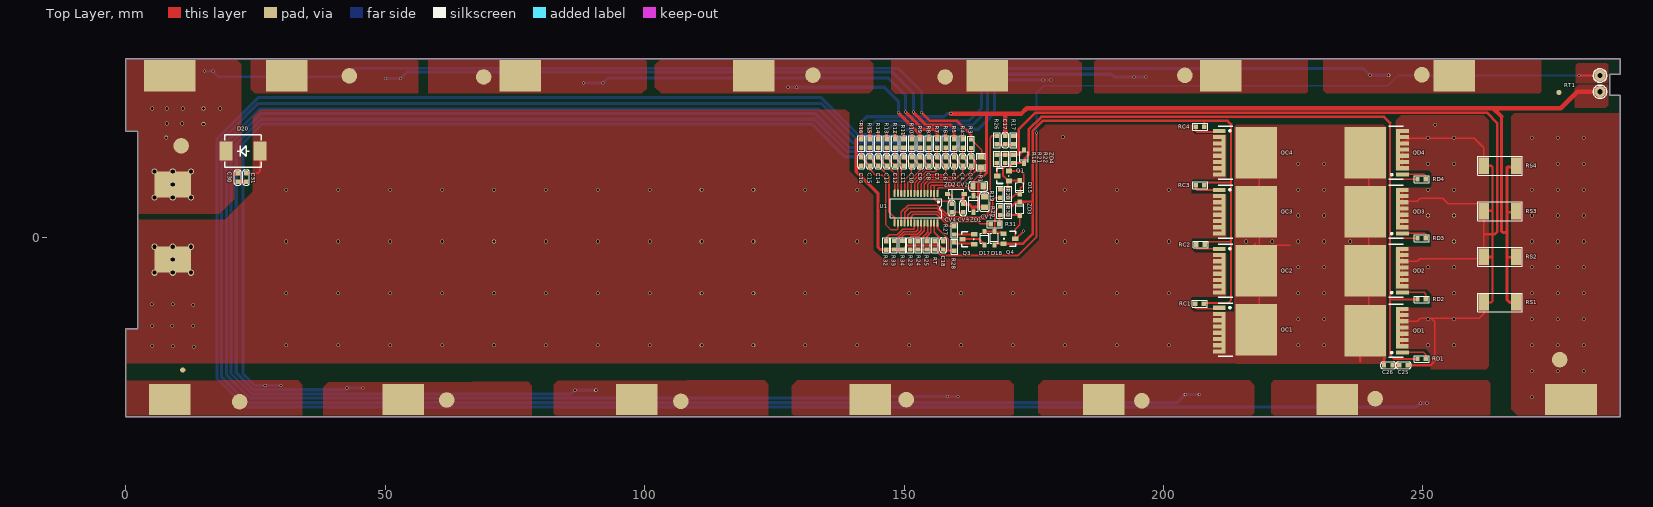
[diagram p0: Top Layer view]
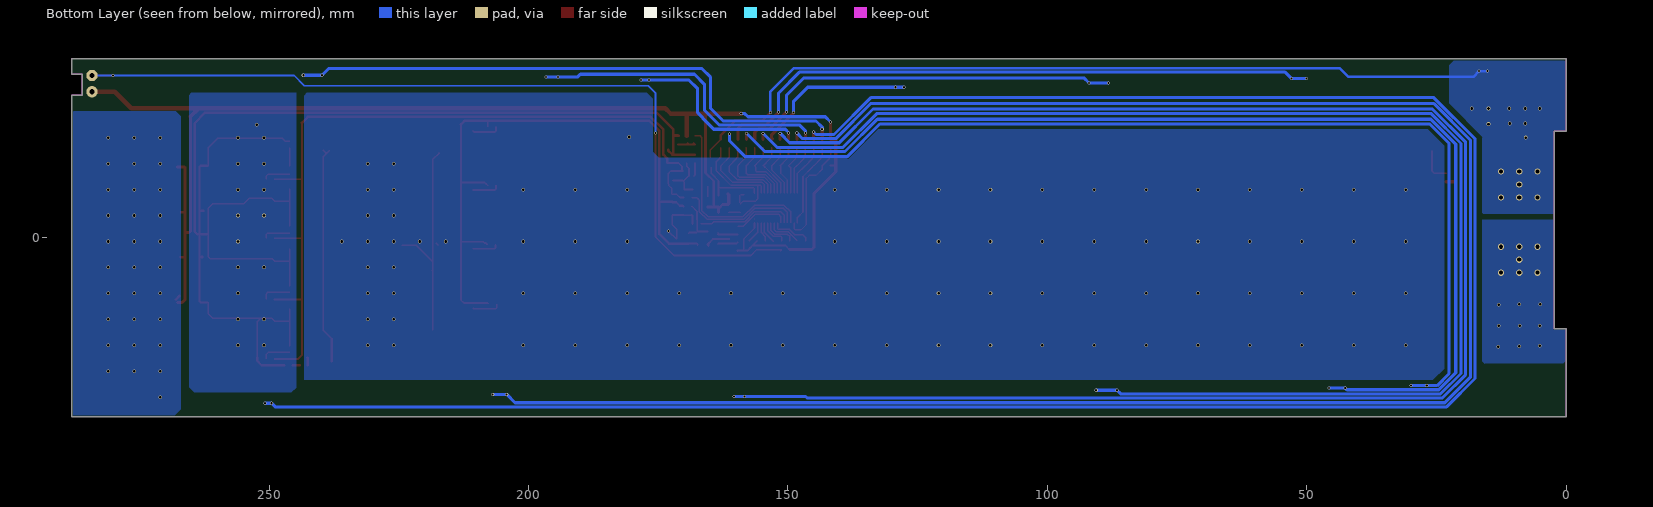
[diagram p1: Bottom Layer view, seen from below]
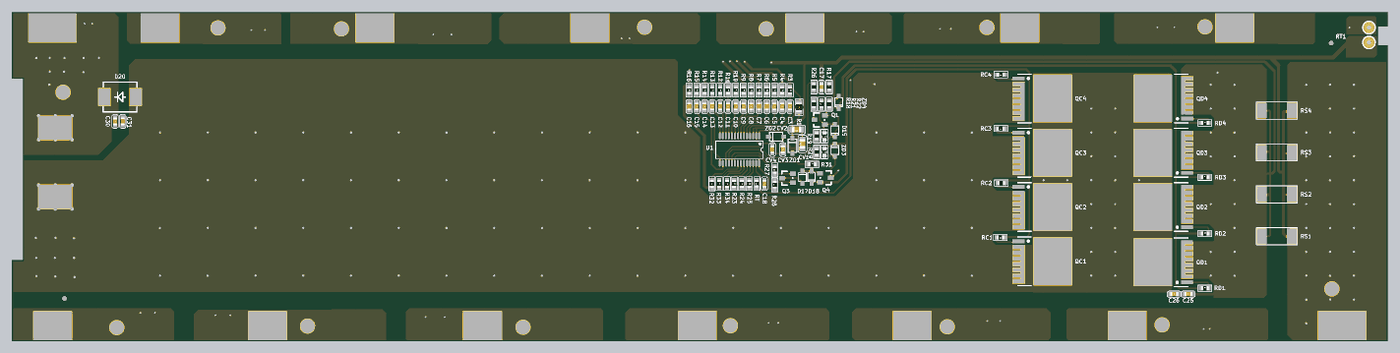
[diagram p2: 3D render of the assembled board from above, using the file's embedded part models]
# Altium PCB MISC84391.PcbDoc
Units mm, origin at the board's own origin, x right, y up, seen from the top; angles counter-clockwise.
Board outline 288 x 69 mm, 2 copper layers (Top Layer, Bottom Layer); 91 components, 64 nets, 309 pads, 210 vias.

## Layer stack, top to bottom (the 12.6 mil dielectric is the usual default, probably not edited)
Top Solder: solder mask 0.0102, Solder Resist, Dk 3.5
Top Layer: signal copper 0.0356
Dielectric 1: dielectric 0.32, FR-4, Dk 4.8
Bottom Layer: signal copper 0.0356
Bottom Solder: solder mask 0.0102, Solder Resist, Dk 3.5

## Board outline
0,-34.5 0,-17.5 2.3,-17.5 2.3,20.5 0,20.5 0,34.5 288,34.5 288,31.5 286,31.5 286,27.5 288,27.5 288,-34.5

## Design rules (kind name [scope] priority, off if disabled: settings)
Clearance [All] p1: gap=0.2 ignorepadtopadclearanceinfootprint=FALSE
ComponentClearance [All] p1: gap=0.2 collisioncheckmode=3 verticalgap=0.254 showdistances=FALSE
PolygonConnect [All] p1: connectstyle=Direct reliefconductorwidth=0.254 reliefentries=4 polygonreliefangle="90 Angle" airgapwidth=0.254
RoutingVias [All] p1: holewidth=0.4 width=0.6 viastyle="Through Hole" minholewidth=0.4 minwidth=0.6 maxholewidth=0.4 maxwidth=0.6
SolderMaskExpansion [All] p1: expansion=0.102 istentingtop=FALSE
SupplyNets "Schematic Supply Nets" [InNet('B-')] p1: voltage=0.000
Width [All] p1: maxlimit=1 minlimit=0.2 preferedwidth=0.25
29 further rules are at their usual default settings.

## Components (designator, comment, footprint, x,y, rotation, side; value= is the part's Value field where it differs from the comment)
C3 "104" CAP0603 162.922,14.7 r0 top
C4 "104" CAP0603 161.295,14.7 r0 top
C5 "104" CAP0603 159.668,14.7 r0 top
C6 "104" CAP0603 158.04,14.7 r0 top
C7 "104" CAP0603 156.413,14.7 r0 top
C8 "104" CAP0603 154.786,14.7 r0 top
C9 "104" CAP0603 153.158,14.7 r0 top
C10 "104" CAP0603 151.531,14.7 r0 top
C11 "104" CAP0603 149.904,14.7 r0 top
C12 "104" CAP0603 148.276,14.7 r0 top
C13 "104" CAP0603 146.649,14.7 r0 top
C14 "104" CAP0603 145.022,14.7 r0 top
C15 "104" CAP0603 143.395,14.7 r0 top
C16 "0.47uF" CAP0603 141.767,14.7 r0 top
C17 "104" CAP0603 169.5,18.8 r180 top
C18 "104" CAP0603 157.55,-1.467 r0 top
C25 "0.1uF" CAP0603 246.255,-24.587 r270 top
C26 "0.1uF" CAP0603 243.32,-24.587 r270 top
C30 "0.1uF" CAP0603 21.6,11.6 r180 top
C31 "0.1uF" CAP0603 23.2,11.6 r0 top
CV1 "2.2uF" CAP0805 165.5,6.9 r90 top
CV2 "2.2uF" CAP0805 164.3,9.9 r180 top
CV3 "0.1uF" CAP0603 161.4,5.7 r0 top
CV4 "0.1uF" CAP0603 159.2,5.7 r180 top
D15 "1N4148" SOD323 172.3,9.7 r270 top
D17 "1N4148" SOD323 165.5,-0.1 r90 top
D18 "1N4148" SOD323 167.4,-0.1 r270 top
D20 "RS3M" SMC 22.625,16.7 r180 top
Q1 "MMBT5401" SOT-23-3 169.1,11.9 r90 top
Q3 "MMBT5401" SOT-23-3 162.4,-0.3 r90 top
Q4 "MMBT5401" SOT-23-3 170.3,-0.2 r270 top
QC1 "NMOS" TOLL_123 214.383,-17.712 r270 top
QC2 "NMOS" TOLL_123 214.383,-6.349 r270 top
QC3 "NMOS" TOLL_123 214.383,5.021 r270 top
QC4 "NMOS" TOLL_123 214.383,16.388 r270 top
QD1 "NMOS" TOLL_123 242.393,-17.912 r90 top
QD2 "NMOS" TOLL_123 242.393,-6.349 r90 top
QD3 "NMOS" TOLL_123 242.393,5.021 r90 top
QD4 "NMOS" TOLL_123 242.422,16.388 r90 top
R1 "2K" RES0805 164.8,15.6 r270 top
R3 "2K" RES0603 162.922,18.1 r0 top
R4 "2K" RES0603 161.277,18.15 r0 top
R5 "2K" RES0603 159.651,18.15 r0 top
R6 "2K" RES0603 158.025,18.15 r0 top
R7 "2K" RES0603 156.399,18.15 r0 top
R8 "2K" RES0603 154.774,18.15 r0 top
R9 "2K" RES0603 153.148,18.15 r0 top
R10 "2K" RES0603 151.522,18.15 r0 top
R11 "2K" RES0603 149.896,18.15 r0 top
R12 "2K" RES0603 148.27,18.15 r0 top
R13 "2K" RES0603 146.645,18.15 r0 top
R14 "2K" RES0603 145.019,18.15 r0 top
R15 "2K" RES0603 143.393,18.15 r0 top
R16 "2K" RES0603 141.767,18.15 r0 top
R17 "1K" RES0603 171.1,18.8 r180 top
R18 "510R" RES0603 167.9,15.19 r180 top
R19 "1K" RES0603 168.5,8.5 r180 top
R20 "NC" RES0603 170.1,8.5 r0 top
R21 "5.1M" RES0603 169.5,15.2 r180 top
R22 "5.1M" RES0603 171.1,15.2 r180 top
R23 "270K" RES0603 151.185,-1.467 r0 top
R24 "41.2K" RES0603 152.776,-1.467 r0 top
R25 "22K" RES0603 154.367,-1.467 r0 top
R26 "10K" RES0603 167.9,18.8 r180 top
R27 "10K" RES0603 159.7,1.41 r180 top
R28 "3M" RES0603 159.7,-1.7 r180 top
R29 "5.1M" RES0603 168.5,5.2 r0 top
R30 "5.1M" RES0603 170.1,5.2 r0 top
R31 "1M" RES0603 167.51,2.6 r90 top
R32 "200K" RES0603 146.55,-1.482 r0 top
R33 "200K" RES0603 148.075,-1.457 r0 top
R34 "499K" RES0603 149.7,-1.457 r0 top
RC1 "47R" RES0603 206.955,-12.712 r270 top
RC2 "47R" RES0603 207.145,-1.312 r270 top
RC3 "47R" RES0603 207.045,10.088 r270 top
RC4 "47R" RES0603 207.055,21.388 r270 top
RD1 "47R" RES0603 249.745,-23.362 r90 top
RD2 "47R" RES0603 249.745,-11.887 r90 top
RD3 "47R" RES0603 249.745,-0.112 r90 top
RD4 "47R" RES0603 249.745,11.263 r90 top
RS1 "" 2512 264.795,-12.462 r90 top
RS2 "" 2512 264.795,-3.687 r90 top
RS3 "" 2512 264.795,5.088 r90 top
RS4 "" 2512 264.795,13.863 r90 top
RT "NC" RES0603 155.959,-1.467 r180 top
RT1 "103AT B=3435" WK 284.092,29.627 r270 top locked
U1 "CW1143" SSOP-28-0.635 152.322,5.7 r270 top locked
ZD1 "68V" SOD123 163.4,6.5 r90 top
ZD2 "68V" SOD123 160,8.4 r180 top
ZD3 "15V" SOD323 172.3,5.6 r90 top
ZD4 "15V" SOD323 173.1,15.6 r270 top

## Footprints (in the part's own frame and the unit in brackets; to place one, negate y for a bottom-side part, rotate by r counter-clockwise, add the part's x,y. Pads: shape width x height; smd on the part's side, far side on the other; paste and mask are expansions set on the pad)
2512 [mm]
  rect 3.2x2 smd: 1(0,3.05) 2(0,-3.15)
  silkscreen extent -1.8,-4.33 1.8,4.25
CAP0603 [mm] "CAP0402"
  rect 0.88x0.83 smd mask+0: 1(0,0.81) 2(0,-0.81)
  silkscreen extent -0.65,-1.45 0.65,1.45, body extent -0.41,-0.79 0.4,0.81, height 0.88
CAP0805 [mil]
  rect 43.31x50 smd: 1(-40,0)
  rect 40x50 smd: 2(40,0)
  silkscreen extent -73,-36 71,36, body extent -39,-25 39,25, height 35
RES0603 [mm] "CAP0402"
  rect 0.88x0.83 smd mask+0: 1(0,0.81) 2(0,-0.81)
  silkscreen extent -0.65,-1.45 0.65,1.45, body extent -0.4,-0.83 0.4,0.77, height 0.3
RES0805 [mil]
  rect 40x50 smd: 1(0,0) 2(80,0)
  silkscreen extent -28,-32 107,32, body extent 1,-25 79,24, height 4
SMC [mm]
  rect 2.44x3.62 smd: 1(-3.275,0) 2(3.275,0)
  silkscreen extent -3.55,-3.1 3.55,3.1
SOD123 [mm]
  rect 1x0.8 smd: 1(-1.6,0) 2(1.6,0)
  silkscreen extent -1.4,-0.9 1.4,0.9
SOD323 [mm]
  rect 1x0.8 smd: 1(-1.3,0) 2(1.3,0)
  silkscreen extent -0.92,-0.8 0.93,0.8
SOT-23-3 [mil]
  rect 36x47.24 smd: 1(-37.5,-43.94) 2(37.5,-43.94) 3(0.5,43.94)
  silkscreen extent -58,-41 58,49
SSOP-28-0.635 [mm]
  rect 1.4x0.4 smd: 1(-2.838,4.127) 28(2.862,4.128)
  oval 1.4x0.4 smd: 2(-2.838,3.492) 3(-2.838,2.857) 4(-2.838,2.222) 5(-2.838,1.587) 6(-2.838,0.952) 7(-2.838,0.317) 8(-2.838,-0.318) 9(-2.838,-0.953) 10(-2.838,-1.588) 11(-2.838,-2.223) 12(-2.838,-2.858) 13(-2.862,-3.493) 14(-2.862,-4.128) 15(2.862,-4.127) 16(2.862,-3.492) 17(2.862,-2.857) 18(2.862,-2.222) 19(2.862,-1.587) 20(2.862,-0.952) 21(2.862,-0.317) 22(2.862,0.318) 23(2.862,0.953) 24(2.862,1.588) 25(2.862,2.223) 26(2.862,2.858) 27(2.862,3.493)
  silkscreen extent -1.79,-4.96 1.86,4.96
TOLL_123 [mm] "贴片MOS"
  rect 0.8x2.5 smd: 1(-4.2,-3.638)
  rect 0.8x1.7 smd: 2(-3,-4) 2(-1.8,-4) 2(-0.6,-4) 2(0.6,-4) 2(1.8,-4) 2(3,-4) 2(4.2,-4)
  rect 8x0.8 smd: 2(0.6,-2.788)
  rect 9.9x8 smd: 3(0,3.5)
  silkscreen extent -5.1,-3.8 5.1,-1
WK [mm]
  round 2.2 hole 1: 1(-1.625,0.025) 2(1.5,0.025)
  silkscreen extent -2.91,-1.27 2.8,1.33

## Part data
C3 C4 C5 C6 C7 C8 C9 C10 C11 C12 C13 C14 C15 C16 C17 C18 C25 C26 C30 C31 CV1 CV2 CV3 CV4: library part CAP
D15 D17 D18 D20: library part DIODE, "DIODE"
Q1 Q3 Q4: library part PNP, "PNP Bipolar Transistor"
R1 R3 R4 R5 R6 R7 R8 R9 R10 R11 R12 R13 R14 R15 R16 R17 R18 R19 R20 R21 R22 R23 R24 R25 R26 R27 R28 R29 R30 R31 R32 R33 R34 RC1 RC2 RC3 RC4 RD1 RD2 RD3 RD4 RS1 RS2 RS3 RS4 RT: library part RES
RT1: library part RT1
ZD1 ZD2 ZD3 ZD4: library part "D Zener", "Zener Diode"

## Free pads (board coordinates)
  round 0.075 on Keep-Out: 1(-10.332,-6.165) 1(79.33,-42.487)
  rect 10x6 smd: 597(278.5,-31.2) 598(8.5,31.2)
  rect 7x5 smd: 598(9.075,-4.233) 598(9.075,10.267)
  rect 8x6 smd: 599(31,31.2) 600(8.5,-31.2) 601(53.5,-31.2) 602(76,31.2) 603(98.5,-31.2) 604(121,31.2) 605(143.5,-31.2) 606(166,31.2) 607(188.5,-31.2) 608(211,31.2) 609(233.5,-31.2) 610(256,31.2)
  round 3 smd: 631(10.7,17.7) 634(43.125,31.175) 635(68.975,30.975) 636(132.45,31.325) 637(157.925,30.975) 638(204.125,31.275) 639(249.8,31.4) 640(276.35,-23.5) 641(240.8,-31.025) 642(195.825,-31.425) 643(150.425,-31.2) 644(107,-31.525) 645(61.875,-31.275) 646(21.95,-31.6)
  round 1 smd: 649(276.2,28) 650(11,-25.5)

## Via types
v1: diameter 0.7, hole 0.5, Top Layer to Bottom Layer, tented both sides, 152 vias
v2: diameter 0.6, hole 0.4, Top Layer to Bottom Layer, tented both sides, 44 vias
v3: diameter 1.2, hole 0.8, Top Layer to Bottom Layer, tented both sides, 14 vias

## Nets (pads, with @x,y where several pads share a name; then routed paths per layer and width w, separated by ;. In a path a pad name is that pad's centre, name@x,y a point inside that pad or via, vN(x,y) a via of type N, cw(c..) or ccw(c..) an arc to the next point about the centre after c; other vN are vias at no path point)
B1: pad.610 pad.639 R15.1 | length 111.1
  Top Layer w0.6: R15.1 143.393,20.893 v2(143.4,20.9)
  Bottom Layer w0.6: v2(143.4,20.9) 143.4,21.3 144.6,22.5 162.5,22.5 164.9,24.9 164.9,30.9 166.6,32.6 238.5,32.6 v2(239.8,31.3) v2(243.4,31.3)
B2: pad.609 pad.641 R14.1 | length 417.4
  Top Layer w0.6: R14.1 145.1,19.041 v2(145.1,20.4)
  Bottom Layer w0.6: v2(145.1,20.4) 144.6,19.9 141.131,19.9 134.031,27 25.537,27 17.6,19.063 17.6,-27.131 23.069,-32.6 248.8,-32.6 v2(249.5,-31.9) v2(250.8,-31.9)
B3: pad.608 pad.638 R13.1 | length 59.3
  Top Layer w0.6: R13.1 v2(146.645,20.155)
  Bottom Layer w0.6: v2(146.645,20.155) 146.645,20.645 147.7,21.7 163.2,21.7 166.1,24.6 166.1,29.6 168,31.5 190,31.5 190.5,31 v2(194.3,31) v2(196.6,31)
B4: pad.607 pad.642 R12.1 | length 374.1
  Top Layer w0.6: R12.1 148.27,20.17 v2(148.3,20.2)
  Bottom Layer w0.6: v2(148.3,20.2) 147.2,19.1 140.8,19.1 134,25.9 25.569,25.9 18.5,18.831 18.5,-26.9 23.4,-31.8 202.6,-31.8 v2(204.2,-30.2) v2(206.9,-30.2)
B5: pad.606 pad.637 R11.1 | length 36.7
  Top Layer w0.6: R11.1 149.896,20.196 v2(149.9,20.2)
  Bottom Layer w0.6: v2(149.9,20.2) 149.9,20.279 150.521,20.9 164.3,20.9 166.4,23 166.4,23.1 167.4,24.1 167.4,28.7 169.1,30.4 v2(176.8,30.4) v2(178.3,30.4)
B6: pad.605 pad.643 R10.1 | length 327.1
  Top Layer w0.6: v2(151.5,20.1) 151.522,20.078 R10.1
  Bottom Layer w0.6: v2(151.5,20.1) 149.7,18.3 140.1,18.3 133.6,24.8 25.806,24.8 19.4,18.394 19.4,-26.394 23.906,-30.9 146.3,-30.9 146.6,-30.6 v2(158.4,-30.6) v2(160.413,-30.6)
B7: pad.604 pad.636 R9.1 | length 31.7
  Top Layer w0.6: v2(148.9,24.1) 153.148,19.852 R9.1 153.033,19.075 R9.1@153.008,19.075
  Bottom Layer w0.6: v2(127.64,29) v2(129.3,29) 146.2,29 148.9,26.3 v2(148.9,24.1)
B8: pad.603 pad.644 R8.1 | length 258.4
  Top Layer w0.6: R8.1 154.8,18.986 v2(154.8,20.1)
  Bottom Layer w0.6: v2(90.6,-29.4) v2(86.6,-29.4) 85.9,-30.1 24.237,-30.1 20.3,-26.163 20.3,18.163 26.037,23.9 132.9,23.9 139.4,17.4 152.1,17.4 v2(154.8,20.1)
B9: pad.602 pad.635 R7.1 | length 76.2
  Top Layer w0.6: v2(150.3,24.2) 153.6,20.9 155.8,20.9 156.399,20.301 R7.1
  Bottom Layer w0.6: v2(88.2,29.8) v2(92,29.8) 93,30.8 146.9,30.8 150.3,27.4 v2(150.3,24.2)
B10: pad.601 pad.645 R6.1 | length 213.8
  Top Layer w0.6: v2(158,20.1) 158.025,20.075 R6.1
  Bottom Layer w0.6: v2(45.7,-29) v2(42.6,-29) 42.3,-29.3 24.569,-29.3 21.3,-26.031 21.3,18.031 26.103,22.834 132.766,22.834 139,16.6 154.5,16.6 v2(158,20.1)
B11: pad.599 pad.634 R5.1 | length 118.8
  Top Layer w0.6: v2(151.8,24.2) 154.3,21.7 159,21.7 159.651,21.049 R5.1
  Bottom Layer w0.6: v2(50.1,30.7) v2(53,30.7) 54.2,31.9 147.8,31.9 151.8,27.9 v2(151.8,24.2)
B12: pad.600 pad.646 R4.1 | length 199.1
  Top Layer w0.6: R4.1 v2(161.277,19.977)
  Bottom Layer w0.6: v2(29.9,-28.5) v2(26.9,-28.5) 24.9,-28.5 22.6,-26.2 22.6,18.2 26.3,21.9 132.3,21.9 138.6,15.6 158.222,15.6 161.277,18.655 v2(161.277,19.977)
B+: C30.2 D20.2 pad.598@8.5,31.2 pad.598@9.075,10.267 pad.631 R1.1 R3.1 | length 161.5
  Top Layer w0.3: R3.1 162.947,18.91 164.975,16.882 R1.1@164.975,15.557
  Top Layer w0.5: v2(153.4,24.1) 155,22.5 160.2,22.5 162.918,19.782 162.918,19.029 R3.1@162.922,19.025
  Bottom Layer w0.5: v2(15.2,32.1) v2(16.8,32.1) 17.9,31 42,31 43.65,32.65 148.9,32.65 153.4,28.15 v2(153.4,24.1)
  other v1: 7.8,19.3 15,21.9 7.9,22 10.9,22 5.1,24.9 7.9,24.9 11,24.9 15,24.9 18.2,24.9
  other v3: 5.575,7.767 9.075,7.767 12.575,7.767 9.075,10.267 5.575,12.767 9.075,12.767 12.575,12.767
B-: C16.2 C17.2 C18.2 CV1.1 CV3.1 pad.597 pad.640 R16.1 R28.1 R32.2 R33.2 R34.2 RS1.2 RS2.2 RS3.2 RS4.2 RT1.2 RT.2 U1.28 ZD1.1 ZD2.1 | length 281
  Top Layer w0.3: U1.28 156.45,1.8 158.5,-0.25 158.5,-2.41 158.444,-2.466
  Top Layer w0.35: R34.2 149.725,-2.267 150.505,-1.487 156.814,-1.487 156.9,-1.573
  Top Layer w0.4: 140.782,14.065 140.957,13.89 C16.2 ; RT.2@155.984,-0.657 156.814,-1.487 ; 156.9,-1.573 157.31,-1.983 157.31,-2.062 C18.2@157.525,-2.277 ; C18.2 157.739,-2.466 158.444,-2.466 159.656,-2.466 R28.1
  Top Layer w0.5: 164.3,5.884 164.3,10.9 165.885,12.485 165.885,23.815 165.8,23.9
  Top Layer w0.6: R16.1 140.782,18.96 140.782,14.065 140.782,12.718 145,8.5 145,-1.9 145.367,-2.267 R34.2 ; R16.1@141.767,19.075 141.767,22.267 v2(141.8,22.3) ; ZD2.1 161.5,8.4 161.4,8.3 CV3.1 161.515,6.395 162.605,6.395 163.4,5.6 ZD1.1 ; 163.4,5.884 164.3,5.884 CV1.1 ; 265.145,23.355 265.145,1.255 265.401,0.999 266.17,0.999 ; RS1.2@267.245,-11.213 RS1.2@267.945,-11.913 ; RS1.2@267.645,-12.487 266.745,-12.487 266.17,-11.912 266.17,0.999 ; RS4.2@267.72,13.638 266.32,13.638 266.17,13.488 266.17,0.999
  Top Layer w0.8: v2(158.995,23.905) 159,23.9 165.8,23.9 169.4,23.9 ; C17.2 169.5,23.8 169.4,23.9 ; 265.145,23.355 263.55,24.95 ; RT1.2 279.727,28.127 276.55,24.95 263.55,24.95 ; 169.4,23.9 172.6,23.9 173.65,24.95 263.55,24.95
  Bottom Layer w0.6: v2(141.8,22.3) 142.8,23.3 157.7,23.3 158.305,23.905 v2(158.995,23.905)
  other v1: 270.978,-30.724 270.978,-25.724 275.978,-25.724 280.978,-25.724 270.978,-20.724 275.978,-20.724 280.978,-20.724 270.978,-15.724 275.978,-15.724 280.978,-15.724 270.978,-10.724 275.978,-10.724 280.978,-10.724 270.978,-5.724 275.978,-5.724 280.978,-5.724 270.978,-0.724 275.978,-0.724 280.978,-0.724 270.978,4.276 275.978,4.276 280.978,4.276 270.978,9.276 275.978,9.276 280.978,9.276 270.978,14.276 275.978,14.276 280.978,14.276 270.978,19.276 275.978,19.276 280.978,19.276
CO: R27.2 U1.20 | length 10.7
  Top Layer w0.25: U1.20 151.37,4.07 151.8,4.5 156.307,4.5 158.587,2.22 R27.2
CS: R26.2 U1.17 | length 36.9
  Top Layer w0.25: U1.17 149.465,4.965 150.8,6.3 156.436,6.3 158.736,4 165.4,4 166.6,5.2 166.6,19.289 166.921,19.61 R26.2 R26.2@168,19.61
DCTL: R32.1 U1.21 | length 7.9
  Top Layer w0.25: R32.1 146.55,-0.032 147.182,0.6 148.7,0.6 149.15,1.05 149.177,1.05 149.727,1.6 151.858,1.6 152.005,1.746 U1.21
DO: R19.1 U1.18 | length 24.6
  Top Layer w0.25: U1.18 150.1,4.9 150.9,5.7 156.4,5.7 158.55,3.55 165.586,3.55 167.05,5.014 167.05,7.25 167.49,7.69 ; 167.59,7.69 R19.1
NetC17_1: C17.1 R17.1 R26.1 | length 4
  Top Layer w0.25: R26.1@167.925,17.99 R26.1@168.215,18.28 ; C17.1@169.185,18.28 C17.1@169.475,17.99
  Top Layer w0.4: R26.1 R26.1@167.925,17.99 ; R26.1@168.025,17.99 169.575,17.99 R17.1@171.2,17.99
NetC18_1: C18.1 U1.27 | length 4.2
  Top Layer w0.25: U1.27 155.815,1.053 157.525,-0.657 C18.1
NetC25_1: C25.1 QD1.2 QD2.2 QD3.2 QD4.2 R17.2 R18.2 R21.2 R22.2 RS1.1 RS2.1 RS3.1 RS4.1 ZD4.1 | length 279
  Top Layer w0.25: QD1.2@246.031,-20.912 QD1.2@246.031,-16.112 ; QD1.2@246.031,-13.712 QD1.2@246.031,-16.112 ; QD2.2@246.031,-9.349 QD2.2@246.031,-4.549 ; QD2.2@246.031,-2.149 QD2.2@246.031,-4.549 ; QD3.2@246.031,2.214 QD3.2@246.031,7.014 ; QD3.2@246.031,9.414 QD3.2@246.031,7.014 ; QD4.2@246.031,13.777 QD4.2@246.031,17.377 ; QD4.2@246.031,18.577 246.901,18.577 247.492,19.169 259.863,19.169 261.745,17.288 RS4.1 ; 252.295,-23 252.295,-16.237 251.578,-15.52 ; RS1.1 261.745,-14.612 260.837,-15.52 251.578,-15.52 ; QD1.2@246.031,-16.112 248.923,-16.112 249.515,-15.52 251.578,-15.52 ; QD2.2@246.031,-4.549 248.923,-4.549 249.515,-3.957 249.621,-4.062 261.37,-4.062 RS2.1 261.745,0.7 RS3.1 261.745,5.688 260.87,6.563 254.863,6.563 253.82,7.606 249.515,7.606 248.923,7.014 QD3.2@246.031,7.014
  Top Layer w0.4: RS1.1 263.161,-12.462 263.395,-12.228 263.395,0.663 263.395,13.628 263.161,13.863 RS4.1 ; 261.745,0.7 261.782,0.663
  Top Layer w0.45: R18.2 167.905,16.005 R21.2@169.6,16.005 ; R21.2 R22.2
  Top Layer w0.5: R22.2 171.11,16 172.3,16 173.1,16.8 ZD4.1 ; R17.2 171.19,19.7 172.1,19.7 ; 172.1,16.293 172.1,19.7 ; C25.1 251.408,-24.587 252.295,-23.7 252.295,-23 ; 261.782,0.663 263.395,0.663 263.795,0.663 264.345,1.213 264.345,22.055 262.3,24.1 175.35,24.1 172.1,20.85 172.1,19.7
  other v1: 250.978,-20.724 255.978,-20.724 250.978,-15.724 255.978,-15.724 255.978,-10.724 250.978,-5.724 255.978,-5.724 255.978,-0.724 250.978,4.276 255.978,4.276 250.978,9.276 255.978,9.276 250.978,14.276 255.978,14.276 250.978,19.276 255.978,19.276 252.4,21.8
NetC25_2: C25.2 C26.1 | length 1.3
  Top Layer w0.5: C26.1 C25.2
NetC30_1: C30.1 C31.2 | length 1.6
  Top Layer w0.6: C30.1 C31.2
NetCV1_2: CV1.2 CV2.1 | length 2
  Top Layer w0.3: CV2.1@165.416,9.9 165.416,8 CV1.2
NetCV3_2: CV3.2 CV4.1 | length 2.2
  Top Layer w0.3: CV4.1 159.205,4.885 161.395,4.885 CV3.2
NetD15_1: D15.1 Q1.1 R19.2 R20.1 R21.1 | length 9.5
  Top Layer w0.35: R19.2@168.4,9.31 170,9.31 170,10.731 Q1.1 ; R21.1 169.49,14.38 169.49,13.75 169.1,13.361 169.1,11.921 170.073,10.948 Q1.1 ; D15.1@172.2,11 170.268,11 Q1.1
NetD15_2: D15.2 Q1.2 R20.2 R22.1 RD1.1 RD2.1 RD3.1 RD4.1 ZD4.2 | length 157.9
  Top Layer w0.3: 243.67,-11.912 243.695,-11.887 ; 243.67,11.288 243.695,11.263
  Top Layer w0.35: R20.2 170.17,7.76 170.86,7.76 171.48,8.38 172.28,8.38 D15.2 172.4,8.5 172.4,9.5 172.963,10.063 172.963,10.232 173.075,10.345 173.075,12.325 172.547,12.853 Q1.2 170.45,13.086 170.45,13.765 171.075,14.39 R22.1 ZD4.2@173.01,14.39 ; 243.67,22.13 243.67,11.288 243.67,-0.112 ; 243.695,-11.887 RD2.1 ; 243.695,11.263 RD4.1 ; RD1.1 244.37,-23.362 243.67,-22.662 243.67,-11.912 243.67,-0.112 ; RD3.1 243.67,-0.112
  Top Layer w0.4: ZD4.2 ZD4.2@173.3,14.5
  Top Layer w0.5: ZD4.2@173.3,14.5 173.3,15.3 174,16 174,20.84 176.46,23.3 242.5,23.3 243.67,22.13
NetD17_1: D17.1 Q3.3 | length 4.9
  Top Layer w0.4: Q3.3 164.5,-0.287 164.5,-0.3 165.5,-1.3 D17.1 ; D17.1@165.3,-1.587 D17.1@165.3,-1.4
NetD17_2: D17.2 D18.1 Q4.1 R29.1 | length 9.1
  Top Layer w0.35: D17.2 D18.1 ; R29.1 168.475,6.01 167.55,5.085 167.55,3.545 167.49,3.485 167.49,1.29 D18.1 ; Q4.1@169.184,0.853 169.036,1 167.6,1 D18.1
NetD18_2: D18.2 Q4.2 R30.1 RC1.1 RC2.1 RC3.1 RC4.1 ZD3.2 | length 124.2
  Top Layer w0.25: RC1.1@207.765,-12.812 RC1.1@207.765,-12.787 ; RC2.1@208.094,-1.248 208.245,-1.097 RC2.1@208.27,-1.097
  Top Layer w0.35: RC1.1 207.877,-12.6 212.423,-12.6 213.02,-12.003 213.02,-0.765 ; 207.8,22.5 207.865,22.435 RC4.1 ; RC3.1 207.855,10.113 208.095,10.353 208.198,10.353 208.48,10.635 213.02,10.635 ; RC2.1 207.955,-1.287 208.195,-1.047 208.423,-1.047 208.705,-0.765 213.02,-0.765 ; 213.02,21.838 213.02,-0.765
  Top Layer w0.4: D18.2 167.4,-1.3 167.6,-1.1 169.132,-1.1 Q4.2 ; R30.1 170.247,6.157 170.857,6.157 171.534,6.834 172.234,6.834 ZD3.2 ; 174.7,6.9 174.8,6.8
  Top Layer w0.5: Q4.2 172.947,-1.152 174.8,0.7 174.8,6.8 174.8,20.6 176.7,22.5 207.8,22.5 212.358,22.5 213.02,21.838 ; ZD3.2 174.7,6.9
NetQ1_3: Q1.3 R18.1 | length 2.5
  Top Layer w0.35: R18.1 167.9,12.097 Q1.3@168.084,11.913
NetQ3_1: Q3.1 R28.2 | length 4
  Top Layer w0.35: R28.2 159.929,-1.119 163.383,-1.119 Q3.1
NetQ3_2: Q3.2 R27.1 | length 3.8
  Top Layer w0.35: R27.1 159.726,0.626 Q3.2@163.49,0.626 ; Q3.2@163.49,0.926 Q3.2@163.516,0.953
NetQC1_1: QC1.1 RC1.2 | length 5.5
  Top Layer w0.25: RC1.2@206.145,-12.812 206.145,-13.554 206.291,-13.7 210.557,-13.7 QC1.1
NetQC2_1: QC2.1 RC2.2 | length 5
  Top Layer w0.35: RC2.2@206.335,-1.412 206.335,-1.962 206.518,-2.146 QC2.1@210.745,-2.146
NetQC3_1: QC3.1 RC3.2 | length 5.2
  Top Layer w0.35: RC3.2 206.235,9.438 206.452,9.221 QC3.1
NetQC4_1: QC4.1 RC4.2 | length 5.4
  Top Layer w0.35: RC4.2 206.245,20.605 206.45,20.4 210.557,20.4 QC4.1
NetQD1_1: QD1.1 RD1.2 | length 5.5
  Top Layer w0.3: QD1.1 250.167,-22.112 250.555,-22.5 RD1.2
NetQD2_1: QD2.1 RD2.2 | length 5.7
  Top Layer w0.25: QD2.1 250.249,-10.549 250.555,-10.855 RD2.2
NetQD3_1: QD3.1 RD3.2 | length 5.4
  Top Layer w0.25: RD3.2 250.555,0.645
  Top Layer w0.3: QD3.1 250.379,0.821 250.555,0.645
NetQD4_1: QD4.1 RD4.2 | length 5.3
  Top Layer w0.25: RD4.2 250.555,11.913
  Top Layer w0.3: QD4.1 250.28,12.188 250.555,11.913
NetR23_1: R23.1 U1.24 | length 5.5
  Top Layer w0.25: R23.1 151.185,0.104 151.331,0.25 152.85,0.25 153.91,1.31 U1.24
NetR23_2: R23.2 R24.2 R25.2 RT1.1 RT.1 | length 168.5
  Top Layer w0.25: R23.2 R23.2@151.21,-2.277 ; R23.2@151.5,-2.567 R23.2@151.21,-2.277 ; RT.1 R25.2 R24.2 R23.2@151.21,-2.277
  Top Layer w0.35: RT.1 155.984,-2.277 157.107,-3.4 172,-3.4 175.55,0.15 v2(175.55,20.2) ; v2(280.048,31.252) RT1.1
  Bottom Layer w0.35: v2(175.55,20.2) 175.55,27.95 176.9,29.3 243.2,29.3 245.152,31.252 RT1.1
NetR24_1: R24.1 U1.25 | length 4.2
  Top Layer w0.25: R24.1 152.801,-0.657 154.545,1.087 U1.25
NetR25_1: R25.1 U1.26 | length 3.8
  Top Layer w0.25: R25.1 154.367,0.21 155.18,1.023 U1.26
NetR33_1: R33.1 U1.22 | length 6.6
  Top Layer w0.25: R33.1@148.194,-0.57 148.194,-0.553 148.39,-0.357 148.407,-0.357 149.914,1.15 152.25,1.15 152.64,1.54 U1.22
NetR34_1: R34.1 U1.23 | length 6.4
  Top Layer w0.25: R34.1 149.7,0.3 150.1,0.7 152.5,0.7 153.275,1.475 U1.23
P-: C26.2 C31.1 D20.1 pad.598@9.075,-4.233 Q4.3 QC1.2 QC1.3 QC2.2 QC2.3 QC3.2 QC3.3 QC4.2 QC4.3 QD1.3 QD2.3 QD3.3 QD4.3 R29.2 R30.2 R31.2 ZD3.1 | length 106.3
  Top Layer w0.25: QD1.3@237.92,-19.458 239.544,-17.834 239.544,15.611 238.845,16.31 QD4.3@238.334,16.821
  Top Layer w0.35: C31.1 25.43,12.41 25.9,12.88 D20.1 ; R31.2@168.41,2.6 168.41,4.3 R29.2 168.545,4.345 R30.2@170.1,4.345 ; R30.2 172.21,4.39 ZD3.1 172.3,2.486 171.416,1.602 Q4.3 171.559,-0.213 172.952,1.181 172.952,1.252 v2(173,1.3) ; QC4.3@217.232,16.31 218.442,15.1 QC2.3@218.442,-4.624 ; QC2.3@217.41,-1.454 217.727,-1.137 217.795,-1.137 ; QC1.3@218.442,-17.756 QC2.3@218.442,-6.389 ; QC2.3@218.56,-6.271 QC2.3@218.442,-6.389 ; 224.41,-1.454 221.612,-1.454 QC2.3@218.442,-4.624 ; QD4.3@238.845,16.31 238.998,16.31 QD4.3@239.544,16.855 ; QC2.3@218.442,-6.389 QC2.3@218.442,-4.624
  Top Layer w0.5: 237.92,-23.837 QD1.3@237.92,-19.458 ; C26.2 242.51,-23.19 242.6,-23.1
  other v1: 13.1,-21 9.1,-20.9 5.1,-20.8 30.978,-20.724 40.978,-20.724 50.978,-20.724 60.978,-20.724 70.978,-20.724 80.978,-20.724 90.978,-20.724 100.978,-20.724 110.978,-20.724 120.978,-20.724 130.978,-20.724 140.978,-20.724 150.978,-20.724 160.978,-20.724 170.978,-20.724 180.978,-20.724 190.978,-20.724 200.978,-20.724 225.978,-20.724 230.978,-20.724 5.1,-17 9,-17 13,-17 225.978,-15.724 230.978,-15.724 13,-12.9 5,-12.8 9.1,-12.8 30.978,-10.724 40.978,-10.724 50.978,-10.724 60.978,-10.724 70.978,-10.724 80.978,-10.724 90.978,-10.724 100.978,-10.724 110.978,-10.724 120.978,-10.724 130.978,-10.724 140.978,-10.724 150.978,-10.724 160.978,-10.724 170.978,-10.724 180.978,-10.724 190.978,-10.724 200.978,-10.724 225.978,-10.724 230.978,-10.724 225.978,-5.724 230.978,-5.724 30.978,-0.724 40.978,-0.724 50.978,-0.724 60.978,-0.724 70.978,-0.724 80.978,-0.724 90.978,-0.724 100.978,-0.724 110.978,-0.724 120.978,-0.724 130.978,-0.724 140.978,-0.724 180.978,-0.724 190.978,-0.724 200.978,-0.724 215.978,-0.724 220.978,-0.724 225.978,-0.724 230.978,-0.724 235.978,-0.724 225.978,4.276 230.978,4.276 30.978,9.276 40.978,9.276 50.978,9.276 60.978,9.276 70.978,9.276 80.978,9.276 90.978,9.276 100.978,9.276 110.978,9.276 120.978,9.276 130.978,9.276 140.978,9.276 180.978,9.276 190.978,9.276 200.978,9.276 225.978,9.276 230.978,9.276 225.978,14.276 230.978,14.276 180.6,19.4
  other v3: 5.575,-6.733 9.075,-6.733 12.575,-6.733 9.075,-4.233 5.575,-1.733 9.075,-1.733 12.575,-1.733
VC0: C15.2 C16.1 R16.2 U1.16 | length 21.6
  Top Layer w0.3: R16.2 C16.1 141.792,15.51 142.057,15.245 142.057,15.202 143.37,13.89 C15.2 143.396,13.888 143.396,13.201 144.597,12 145.847,12 146.5,11.347 146.5,2.472 147.472,1.5 148.654,1.5 148.83,1.676 U1.16
VC1: C14.2 C15.1 R15.2 U1.15 | length 16.5
  Top Layer w0.3: C15.1 143.42,15.51 143.685,15.245 143.685,15.202 144.997,13.89 C14.2 145.047,13.89 145.312,13.625 145.312,13.6 147.097,11.815 147.097,4.95 148.195,3.852 U1.15 ; C15.1@143.394,15.511 R15.2
VC2: C13.2 C14.1 R14.2 U1.14 | length 10.1
  Top Layer w0.3: R14.2 145.02,17.339 145.02,15.512 C14.1 145.047,15.51 145.312,15.245 145.312,15.202 146.624,13.89 C13.2 146.674,13.89 148.195,12.369 U1.14
VC3: C12.2 C13.1 R13.2 U1.13 | length 9.7
  Top Layer w0.3: R13.2 146.647,17.338 146.647,15.512 C13.1 146.674,15.51 146.939,15.245 146.939,15.202 148.251,13.89 C12.2 148.301,13.89 148.83,13.362 U1.13
VC4: C11.2 C12.1 R12.2 U1.12 | length 9.7
  Top Layer w0.3: R12.2 148.273,17.337 148.273,15.513 C12.1 148.301,15.51 148.566,15.245 148.566,15.202 C11.2@149.879,13.89 ; U1.12 149.465,13.476 C11.2@149.879,13.89 ; C11.2 C11.2@149.879,13.89
VC5: C10.2 C11.1 R11.2 U1.11 | length 10.1
  Top Layer w0.3: R11.2 149.9,17.336 149.9,15.514 C11.1 149.929,15.51 150.194,15.245 150.194,15.202 151.506,13.89 C10.2 151.347,13.706 151.347,12.375 150.1,11.127 U1.11
VC6: C9.2 C10.1 R10.2 U1.10 | length 10.5
  Top Layer w0.3: U1.10 150.735,10.652 153.108,13.025 153.108,13.84 C9.2 153.133,13.89 151.821,15.202 151.821,15.245 151.556,15.51 C10.1 151.527,15.515 151.527,17.336 R10.2
VC7: C8.2 C9.1 R9.2 U1.9 | length 11
  Top Layer w0.3: U1.9 151.37,10.58 154.415,13.625 154.521,13.625 C8.2 ; R9.2 153.153,17.335 153.153,15.515 C9.1 153.183,15.51 153.448,15.245 153.448,15.202 C8.2@154.761,13.89
VC8: C7.2 C8.1 R8.2 U1.8 | length 12.3
  Top Layer w0.3: U1.8@152.09,8.6 152.09,10.592 154.172,12.675 155.996,12.675 156.172,12.851 156.172,13.649 C7.2 156.388,13.89 156.123,14.155 156.123,14.198 154.811,15.51 C8.1 154.78,15.516 154.78,17.334 R8.2
VC9: C6.2 C7.1 R7.2 U1.7 | length 13.8
  Top Layer w0.3: U1.7 152.64,10.435 154.379,12.175 157.8,12.175 158.04,12.416 C6.2 158.015,13.89 157.75,14.155 157.75,14.198 156.438,15.51 C7.1 156.406,15.517 156.406,17.333 R7.2
VC10: C5.2 C6.1 R6.2 U1.6 | length 15
  Top Layer w0.3: U1.6 153.275,10.363 154.586,11.675 159.413,11.675 159.668,11.93 C5.2 159.643,13.89 159.378,14.155 159.378,14.198 158.065,15.51 C6.1 158.033,15.518 158.033,17.333 R6.2
VC11: C4.2 C5.1 R5.2 U1.5 | length 15.5
  Top Layer w0.3: U1.5 153.91,10.291 154.793,11.175 159.789,11.175 161.295,12.681 C4.2 161.27,13.89 159.958,15.202 159.958,15.245 159.693,15.51 C5.1 159.659,15.518 159.659,17.332 R5.2
VC12: C3.2 C4.1 R4.2 U1.4 | length 16.3
  Top Layer w0.3: U1.4 154.545,10.219 155.001,10.675 160.697,10.675 162.922,12.9 C3.2 162.897,13.89 162.632,14.155 162.632,14.198 161.32,15.51 C4.1 161.286,15.519 161.286,17.331 R4.2
VC13: C3.1 CV4.2 R3.2 U1.2 U1.3 ZD2.2 | length 24.9
  Top Layer w0.3: U1.3 155.18,9.974 155.355,10.15 155.847,10.15 ; ZD2.2 158.55,8.25 159.124,8.25 159.3,8.074 CV4.2@159.3,6.7 ; CV4.2@159.1,6.5 159.1,6.585 158.691,6.994 156.308,6.994 155.815,7.488 U1.2 155.815,10.118 155.847,10.15 ; R3.2 162.922,15.51 162.947,15.51 163.8,14.657 163.8,12.883 161.067,10.15 155.847,10.15
VDD: CV2.2 R1.2 U1.1 ZD1.2 | length 14.1
  Top Layer w0.3: U1.1 156.459,8.547 156.459,9.465 156.644,9.65 163.134,9.65 163.384,9.9 163.384,10.984 164.8,12.4 R1.2
  Top Layer w0.4: CV2.2@163.384,9.9 163.392,9.892 163.392,8.108 ZD1.2
VM: R31.1 U1.19 | length 18.8
  Top Layer w0.25: U1.19 150.735,4.3 151.435,5 156.464,5 158.364,3.1 164.3,3.1 164.7,2.7 166.69,2.7 R31.1@166.79,2.6

## Polygon pours and split planes (outlines as drawn)
NetR23_2 on Top Layer "NETR23_2_L01_P093" (solid, remove dead copper, pour order 93): 285.5,29.8 285.7,30 285.7,33.3 285.4,33.6 279.8,33.6 279.4,33.2 279.4,29.8
B- on Top Layer "B-_L01_P092" (solid, pour order 92): 285.745,29.355 285.745,25.545 285.2,25 279.3,25 279.3,28.9 279.9,29.5 285.6,29.5
P- on Top Layer "NONET_L-01_P-001" (solid, remove dead copper, pour order 42): 144.1,-2.3 145.9,-4.1 172.4,-4.1 176.1,-0.4 176.1,20.6 177.3,21.8 205.4,21.8 205.6,21.6 205.6,20.4 206.1,19.9 212,19.9 212.063,19.837 212.063,11.238 205.763,11.238 205.363,10.837 205.363,8.612 205.475,8.5 211.914,8.5 212.113,8.301 212.113,-0.138 205.625,-0.138 205.363,-0.4 205.363,-2.163 206.113,-2.912 211.956,-2.912 212.113,-3.069 212.113,-11.412 205.563,-11.412 205.288,-11.688 205.288,-13.688 205.912,-14.312 211.993,-14.312 213.812,-14.312 218,-18.5 218.3,-18.5 218.3,-24.2 0,-24.2 0,2.3 1.2,3.5 19.1,3.5 24.5,8.9 24.5,23.3 25.9,24.7 138.8,24.7 139.4,24.1 139.4,12.9 144.1,8.2
B- on Top Layer "B-_L01_P088" (solid, pour order 88): 267,-15.2 267,-33.1 268.4,-34.5 288,-34.5 288,24 267.6,24 267,23.4
B6 on Top Layer "NONET_L-01_P-001" (solid, remove dead copper, pour order 84): 129.387,-27.513 128.4,-28.5 128.4,-33.9 128.888,-34.388 152.337,-34.388 152.35,-34.4 170.5,-34.4 170.55,-34.45 170.65,-34.45 171.1,-34 171.1,-28.3 170.3,-27.5 170.287,-27.513
B2 on Top Layer "NONET_L-01_P-001" (solid, remove dead copper, pour order 86): 242.8,-27.515 221.285,-27.515 220.8,-28 220.8,-33.8 221.388,-34.388 242.337,-34.388 242.35,-34.4 262.6,-34.4 263,-34 263,-28.013 262.5,-27.513 243.162,-27.513
B4 on Top Layer "NONET_L-01_P-001" (solid, remove dead copper, pour order 85): 176.787,-27.513 175.9,-28.4 175.9,-33.7 176.588,-34.388 197.337,-34.388 197.35,-34.4 216.9,-34.4 217.5,-33.8 217.5,-28.4 216.613,-27.513
B8 on Top Layer "NONET_L-01_P-001" (solid, remove dead copper, pour order 83): 105.902,-27.529 83.271,-27.529 82.5,-28.3 82.5,-33.9 82.988,-34.388 107.337,-34.388 107.35,-34.4 123.8,-34.4 123.8,-28.2 123.113,-27.513 108.162,-27.513
B12 on Top Layer "NONET_L-01_P-001" (solid, remove dead copper, pour order 82): 16.702,-27.523 0.277,-27.523 -0.1,-27.9 -0.1,-34.1 0.188,-34.388 17.337,-34.388 17.35,-34.4 34,-34.4 34,-28.3 33.3,-27.513 18.162,-27.513
B+ on Top Layer "B+_L01_P081" (solid, pour order 81): 2.3,4.6 2.2,4.7 2.2,20.4 2.3,20.5 0,20.5 0,34.5 21.2,34.5 22.3,33.4 22.3,12.2 22,11.9 20.9,11.9 20.9,7.4 18.1,4.6
B7 on Top Layer "NONET_L-01_P-001" (solid, remove dead copper, pour order 80): 103.188,27.812 102,29 102,33.3 103.264,34.564 114.1,34.564 114.1,34.565 130.762,34.687 142.913,34.687 144.1,33.5 144.1,28.6 143.3,27.8 129.95,27.8 129.937,27.812
B3 on Top Layer "NONET_L-01_P-001" (solid, remove dead copper, pour order 79): 186.888,27.812 186.7,28 186.7,33.9 187.4,34.6 187.436,34.564 204.1,34.564 204.1,34.565 220.762,34.687 227.8,34.687 227.8,28.1 227.5,27.8 219.95,27.8 219.937,27.812
B1 on Top Layer "NONET_L-01_P-001" (solid, remove dead copper, pour order 78): 231.388,27.812 230.8,28.4 230.8,34.4 230.7,34.5 230.764,34.564 249.1,34.564 249.1,34.565 265.762,34.687 272.8,34.687 272.8,28.1 272.5,27.8 264.95,27.8 264.937,27.812
B9 on Top Layer "NONET_L-01_P-001" (solid, remove dead copper, pour order 77): 99.5,27.8 100.4,28.7 100.4,34 99.713,34.687 85.762,34.687 69.1,34.565 58.6,34.565 58.288,34.268 58.288,27.812 84.937,27.812 84.95,27.8
B5 on Top Layer "NONET_L-01_P-001" (solid, remove dead copper, pour order 76): 183.612,27.712 184.2,28.3 184.2,33.6 183.213,34.587 175.562,34.587 158.9,34.465 155.235,34.465 155.2,34.429 147.871,34.429 147.8,34.5 147.5,34.2 147.5,28.5 148.288,27.712
B11 on Top Layer "NONET_L-01_P-001" (solid, remove dead copper, pour order 75): 56.4,27.8 56.4,34 55.713,34.687 40.762,34.687 24.1,34.565 24.1,34.564 24.1,28.6 24.9,27.812 39.937,27.812 39.95,27.8
B10 on Top Layer "NONET_L-01_P-001" (solid, remove dead copper, pour order 47): 78.1,-34.5 78.3,-34.3 78.3,-28.5 77.6,-27.8 66.925,-27.8 66.913,-27.812 39.088,-27.812 38.1,-28.8 38.1,-34.4 38.387,-34.687 43.738,-34.687 67.463,-34.512 67.475,-34.5
P- on Top Layer "NONET_L-01_P-001" (solid, remove dead copper, pour order 41): 241.93,-24.3 242.893,-23.338 242.893,21.309 242.922,21.338 242.459,21.8 214,21.8 213.6,21.4 213.6,-24 214,-24.3
NetC25_1 on Top Layer "NONET_L-01_P-001" (solid, remove dead copper, pour order 40): 251.075,13 251.65,12.425 251.65,10.05 251.275,9.675 245,9.675 244.825,9.5 244.825,1.5 244.9,1.425 251.037,1.425 251.6,0.863 251.6,-1.7 251.55,-1.75 244.975,-1.75 244.8,-1.925 244.8,-10.1 247.15,-10.1 247.275,-9.975 247.275,-9.949 250.736,-9.949 251.675,-10.888 251.675,-13.35 251.5,-13.525 245.075,-13.525 244.825,-13.775 244.825,-21.4 250.525,-21.4 251.55,-22.425 251.55,-25.35 262.15,-25.35 262.7,-24.8 262.7,22.6 261.725,23.575 245.8,23.575 244.8,22.575 244.8,13
P- on Bottom Layer "P-_L02_P095" (solid, pour order 95): 2.3,-17.3 2.3,3.5 16.2,3.5 16.2,-23.8 15.7,-24.3 15.6,-24.2 0.6,-24.2 -0.3,-23.3 -0.1,-23.1 -0.1,-17.5 2.1,-17.5
B+ on Bottom Layer "B+_L02_P094" (solid, pour order 94): 16,4.6 16.2,4.8 16.2,19.3 16.1,19.4 22.6,25.9 22.6,29.3 22.6,33.2 21.7,34.1 0.4,34.1 0,34.5 0,20.5 2.3,20.5 2.3,4.9 2.6,4.6
P- on Bottom Layer "P-_L02_P091" (solid, pour order 91): 26.7,20.9 23.5,17.7 23.5,-25.281 25.731,-27.4 243.2,-27.4 243.2,27.4 242.7,27.9 177.2,27.9 176.1,26.8 176.1,16.6 174.9,15.4 138.1,15.4 132.6,20.9
NetC25_1 on Bottom Layer "NONET_L-01_P-001" (solid, remove dead copper, pour order 90): 244.8,27.9 265,27.9 265.4,27.5 265.4,-28.8 264.4,-29.8 245.7,-29.8 244.8,-28.9
B- on Bottom Layer "B-_L02_P089" (solid, pour order 89): 267,-15.2 267,-33.1 268.4,-34.5 288,-34.5 288,24 287.6,24.4 268,24.4 267,23.4

## Keep-outs
Keep-Out Layer:
  lines w0.1: 0,-34.5 0,-17.5 2.3,-17.5 2.3,20.5 0,20.5 0,34.5 288,34.5 288,31.5 286,31.5 286,27.5 288,27.5 288,-34.5 230.6,-34.5 0,-34.5

## Other copper
Top Layer:
  region net B-: 267.145,5.138 266.245,5.138 266.245,4.688 267.145,4.688
  region net NetC25_1: 263.37,5.463 262.445,5.463 262.445,4.963 263.37,4.963
  region net NetC25_1: 263.345,-3.437 262.645,-3.437 262.645,-4.037 263.345,-4.037
  region net B-: 267.245,-3.537 266.27,-3.537 266.27,-3.962 267.245,-3.962
  rectangle net B-: 156.272,3.5 156.647,3.7

## Silkscreen, mask and mechanical layers (free items; w line width, h text height)
Mechanical 1:
  lines w0.013: -20.694,-4.233 12.575,-4.233 ; -18.315,10.267 12.575,10.267 ; 3.5,31.2 260,31.2 ; 4.5,-31.2 237.5,-31.2 301.423,-31.2 ; 8.5,-56.038 8.5,-28.2 ; 8.5,28.2 8.5,55.143 ; 9.075,-6.233 9.075,12.767 ; 31,28.2 31,55.079 ; 53.5,-52.889 53.5,-28.2 ; 76,28.2 76,54.181 ; 98.5,-47.893 98.5,-28.2 ; 121,28.2 121,51.634 ; 143.5,-49.879 143.5,-28.2 ; 166,28.2 166,50.591 ; 188.5,-48.628 188.5,-28.2 ; 211,28.2 211,56.326 ; 233.5,-45.957 233.5,-28.2 ; 256,28.2 256,46.942 ; 278.5,-42.454 278.5,-27.2 ; 278.5,-34.2 278.5,-7.257 ; 283.101,29.627 292.821,29.627 ; 284.092,27.809 284.092,31.446 ; 283.101,27.809 285.082,27.809 285.082,31.446 283.101,31.446 283.101,27.809
  lines w0.1: -9.6,-22.5 290.4,-22.5 ; -2.6,22.5 297.4,22.5
  text "B1" at 253.774,38.344 h3.3
  text "B9" at 72.799,37.455 h3.3
  text "B+" at 6.505,36.566 h3.3
  text "B11" at 28.095,36.566 h3.3
  text "B7" at 117.249,35.931 h3.3
  text "B5" at 162.588,35.931 h3.3
  text "B3" at 207.038,35.55 h3.3
  text "NTC" at 289.842,28.184 h3.3
  text "CO" at 185.65,-24.525 h2
  text "B6" at 141.125,-38.999 h3.3
  text "B2" at 232.184,-38.999 h3.3
  text "B-" at 277.142,-39.507 h3.3
  text "B12" at 4.473,-39.634 h3.3
  text "B10" at 49.939,-40.015 h3.3
  text "B8" at 96.04,-40.015 h3.3
  text "B4" at 185.321,-40.269 h3.3